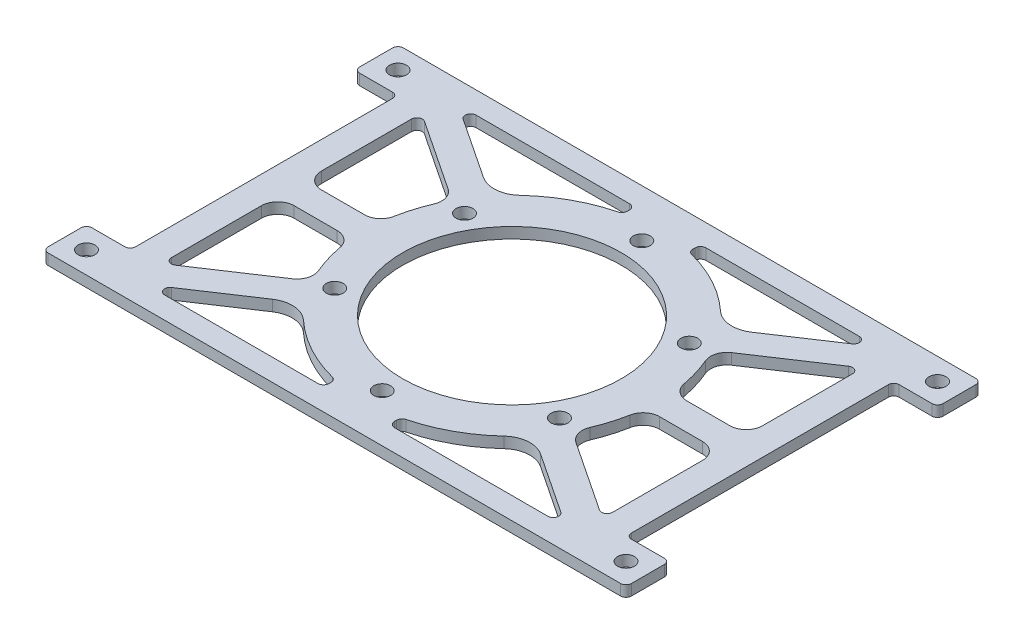
from build123d import *

# Parameters (mm, degrees)
SKETCH_1_R      = 1.55
SKETCH_1_R_2    = 20
EXTRUDE_1_DEPTH = 2
FILLET_1_R      = 1
FILLET_2_R      = 3
FILLET_3_R      = 5


with BuildPart() as part:
    # 草图1 → 凸台-拉伸1 (new body)
    with BuildSketch(Plane(origin=(0, 0, 0), x_dir=(1, 0, 0), z_dir=(0, 1, 0))):
        Polygon((-53.363448016, 32.5), (53.363448016, 32.5), (53.363448016, 24.5), (45.363448016, 24.5), (45.363448016, -24.5), (53.363448016, -24.5), (53.363448016, -32.5), (-53.363448016, -32.5), (-53.363448016, -24.5), (-45.363448016, -24.5), (-45.363448016, 24.5), (-53.363448016, 24.5), align=None)
        with Locations(Location((49.363448016, 28.5, 0), (0, 0, 270))):
            Circle(SKETCH_1_R, mode=Mode.SUBTRACT)
        with Locations(Location((49.363448016, -28.5, 0), (0, 0, 270))):
            Circle(SKETCH_1_R, mode=Mode.SUBTRACT)
        with Locations(Location((-49.363448016, 28.5, 0), (0, 0, 270))):
            Circle(SKETCH_1_R, mode=Mode.SUBTRACT)
        with Locations(Location((-49.363448016, -28.5, 0), (0, 0, 270))):
            Circle(SKETCH_1_R, mode=Mode.SUBTRACT)
        with Locations(Location((20.56810334, 11.875, 0), (0, 0, 270))):
            Circle(SKETCH_1_R, mode=Mode.SUBTRACT)
        with Locations(Location((0, 0, 0), (0, 0, 270))):
            Circle(SKETCH_1_R_2, mode=Mode.SUBTRACT)
        with Locations(Location((20.56810334, -11.875, 0), (0, 0, 270))):
            Circle(SKETCH_1_R, mode=Mode.SUBTRACT)
        with Locations(Location((0, -23.75, 0), (0, 0, 270))):
            Circle(SKETCH_1_R, mode=Mode.SUBTRACT)
        with Locations(Location((-20.56810334, -11.875, 0), (0, 0, 270))):
            Circle(SKETCH_1_R, mode=Mode.SUBTRACT)
        with Locations(Location((-20.56810334, 11.875, 0), (0, 0, 270))):
            Circle(SKETCH_1_R, mode=Mode.SUBTRACT)
        with Locations(Location((0, 23.75, 0), (0, 0, 270))):
            Circle(SKETCH_1_R, mode=Mode.SUBTRACT)
        with BuildLine():
            Line((-38.363448016, 28.5), (-6, 28.5))
            Line((-6, 28.5), (-6, 26.324893162))
            ThreePointArc((-6, 26.324893162), (-14.291214103, 22.907666827), (-21.005853084, 16.963317371))
            Line((-21.005853084, 16.963317371), (-38.363448016, 28.5))
        make_face(mode=Mode.SUBTRACT)
        with BuildLine():
            Line((-23.773530472, 12.799189385), (-40.363448016, 23.825637134))
            Line((-40.363448016, 23.825637134), (-40.363448016, 2.5))
            Line((-40.363448016, 2.5), (-26.884010118, 2.5))
            ThreePointArc((-26.884010118, 2.5), (-25.846952047, 7.806091843), (-23.773530472, 12.799189385))
        make_face(mode=Mode.SUBTRACT)
        with BuildLine():
            Line((-38.363448016, -28.5), (-6, -28.5))
            Line((-6, -28.5), (-6, -26.324893162))
            ThreePointArc((-6, -26.324893162), (-14.291214103, -22.907666827), (-21.005853084, -16.963317371))
            Line((-21.005853084, -16.963317371), (-38.363448016, -28.5))
        make_face(mode=Mode.SUBTRACT)
        with BuildLine():
            Line((-23.773530472, -12.799189385), (-40.363448016, -23.825637134))
            Line((-40.363448016, -23.825637134), (-40.363448016, -2.5))
            Line((-40.363448016, -2.5), (-26.884010118, -2.5))
            ThreePointArc((-26.884010118, -2.5), (-25.846952047, -7.806091843), (-23.773530472, -12.799189385))
        make_face(mode=Mode.SUBTRACT)
        with BuildLine():
            Line((38.363448016, -28.5), (21.005853084, -16.963317371))
            ThreePointArc((21.005853084, -16.963317371), (14.291214103, -22.907666827), (6, -26.324893162))
            Line((6, -26.324893162), (6, -28.5))
            Line((6, -28.5), (38.363448016, -28.5))
        make_face(mode=Mode.SUBTRACT)
        with BuildLine():
            Line((23.773530472, -12.799189385), (40.363448016, -23.825637134))
            Line((40.363448016, -23.825637134), (40.363448016, -2.5))
            Line((40.363448016, -2.5), (26.884010118, -2.5))
            ThreePointArc((26.884010118, -2.5), (25.846952047, -7.806091843), (23.773530472, -12.799189385))
        make_face(mode=Mode.SUBTRACT)
        with BuildLine():
            Line((40.363448016, 2.5), (26.884010118, 2.5))
            ThreePointArc((26.884010118, 2.5), (25.846952047, 7.806091843), (23.773530472, 12.799189385))
            Line((23.773530472, 12.799189385), (40.363448016, 23.825637134))
            Line((40.363448016, 23.825637134), (40.363448016, 2.5))
        make_face(mode=Mode.SUBTRACT)
        with BuildLine():
            Line((38.363448016, 28.5), (21.005853084, 16.963317371))
            ThreePointArc((21.005853084, 16.963317371), (14.291214103, 22.907666827), (6, 26.324893162))
            Line((6, 26.324893162), (6, 28.5))
            Line((6, 28.5), (38.363448016, 28.5))
        make_face(mode=Mode.SUBTRACT)
    extrude(amount=EXTRUDE_1_DEPTH)

    # 圆角1
    fillet_1_edges = [part.edges().sort_by_distance(p)[0] for p in [
        (38.363448016, 1, -28.5),
        (6, 1, -28.5),
        (6, 1, -26.324893162),
        (40.363448016, 1, -23.825637134),
        (40.363448016, 1, 23.825637134),
        (6, 1, 28.5),
        (38.363448016, 1, 28.5),
        (6, 1, 26.324893162),
        (-38.363448016, 1, 28.5),
        (-6, 1, 28.5),
        (-6, 1, 26.324893162),
        (-40.363448016, 1, 23.825637134),
        (-6, 1, -28.5),
        (-38.363448016, 1, -28.5),
        (-6, 1, -26.324893162),
        (-40.363448016, 1, -23.825637134),
        (53.363448016, 1, -32.5),
        (53.363448016, 1, -24.5),
        (45.363448016, 1, -24.5),
        (45.363448016, 1, 24.5),
        (53.363448016, 1, 24.5),
        (53.363448016, 1, 32.5),
        (-53.363448016, 1, 32.5),
        (-53.363448016, 1, 24.5),
        (-45.363448016, 1, 24.5),
        (-45.363448016, 1, -24.5),
        (-53.363448016, 1, -24.5),
        (-53.363448016, 1, -32.5),
    ]]
    fillet(fillet_1_edges, radius=FILLET_1_R)

    # 圆角2
    fillet_2_edges = [part.edges().sort_by_distance(p)[0] for p in [
        (40.363448016, 1, -2.5),
        (23.773530472, 1, -12.799189385),
        (26.884010118, 1, -2.5),
        (40.363448016, 1, 2.5),
        (26.884010118, 1, 2.5),
        (23.773530472, 1, 12.799189385),
        (-40.363448016, 1, 2.5),
        (-23.773530472, 1, 12.799189385),
        (-26.884010118, 1, 2.5),
        (-40.363448016, 1, -2.5),
        (-26.884010118, 1, -2.5),
        (-23.773530472, 1, -12.799189385),
    ]]
    fillet(fillet_2_edges, radius=FILLET_2_R)

    # 圆角3
    fillet_3_edges = [part.edges().sort_by_distance(p)[0] for p in [
        (21.005853084, 1, -16.963317371),
        (21.005853084, 1, 16.963317371),
        (-21.005853084, 1, 16.963317371),
        (-21.005853084, 1, -16.963317371),
    ]]
    fillet(fillet_3_edges, radius=FILLET_3_R)


solid = part.part
